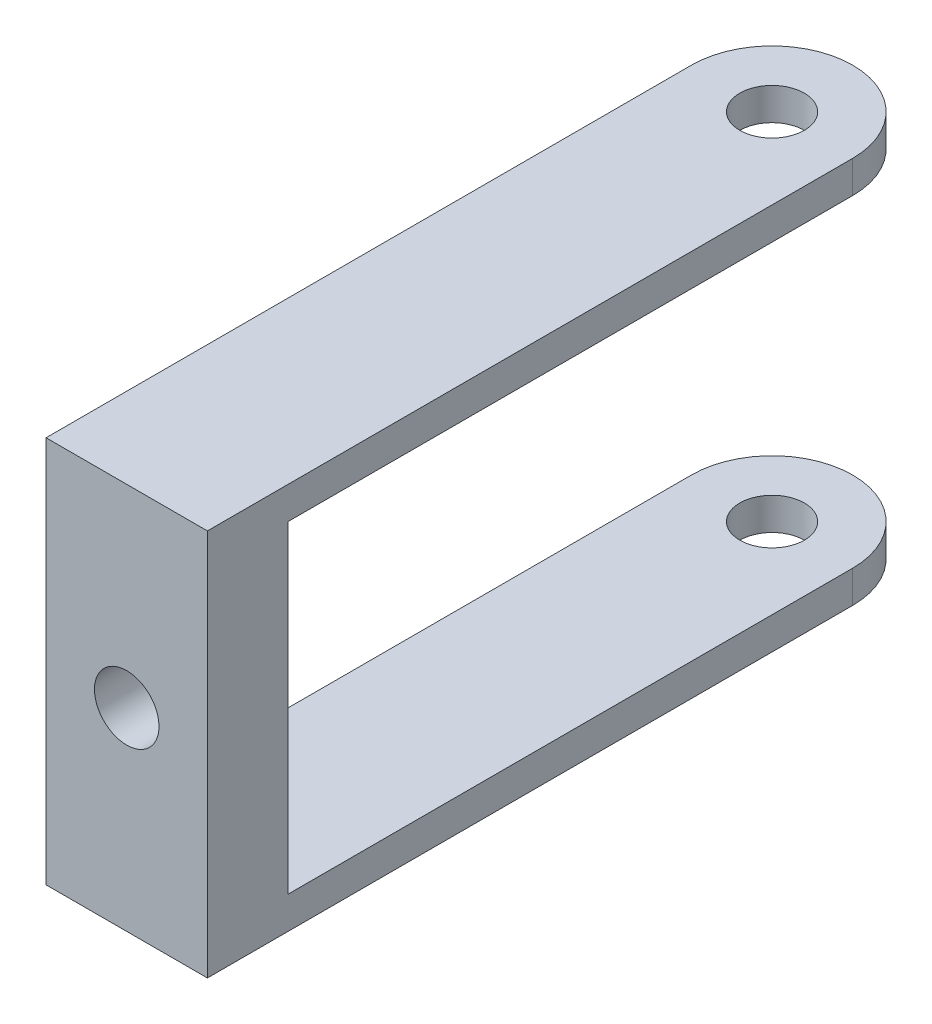
SolidWorks part; units mm, degrees
ref_plane "Front Plane" through (0, 0, 0) normal (0, 0, 1) x (1, 0, 0)
ref_plane "Top Plane" through (0, 0, 0) normal (0, 1, 0) x (1, 0, 0)
ref_plane "Right Plane" through (0, 0, 0) normal (1, 0, 0) x (0, 0, -1)
other "Configuration Table"
sketch "Sketch1" plane through (0, 0, 0) normal (0, 1, 0) x (1, 0, 0)
  line L0 (-5, 0) -> (-5, -40)
  line L1 (0, -3.85) -> (0, 3.85) construction
  line L2 (5, 0) -> (5, -40)
  line L3 (-5, -40) -> (5, -40)
  arc A0 (5, 0) -> (-5, 0) centre (0, 0) ccw
  dimension "D1" = 10
  dimension "D2" = 40
extrude "Boss-Extrude1" add sketch "Sketch1" along normal blind 24
sketch "Sketch2" plane through (0, 24, 0) normal (0, 1, 0) x (1, 0, 0)
  circle A0 centre (0, 0) radius 2
  dimension "D1" = 4
extrude "Cut-Extrude1" cut sketch "Sketch2" against normal through all both and the other way through all
sketch "Sketch3" plane through (5, 0, 0) normal (1, 0, 0) x (0, 0, -1)
  line L0 (-35, 22) -> (5, 22)
  line L1 (5, 0) -> (5, 24) construction
  line L2 (5, 22) -> (5, 2)
  line L3 (5, 2) -> (-35, 2)
  line L4 (-35, 2) -> (-35, 22)
  line L5 (-40, 24) -> (0, 24) construction
  line L6 (-40, 0) -> (0, 0) construction
  line L7 (-40, 24) -> (-40, 0) construction
  dimension "D1" = 2
  dimension "D2" = 2
  dimension "D3" = 5
extrude "Cut-Extrude2" cut sketch "Sketch3" against normal through all
sketch "Sketch4" plane through (0, 0, 35) normal (0, 0, -1) x (-1, 0, 0)
  line L0 (0, 24) -> (0, 0) construction
  line L1 (5, 24) -> (-5, 24) construction
  circle A0 centre (0, 12) radius 2
  dimension "D1" = 4
extrude "Cut-Extrude3" cut sketch "Sketch4" against normal through all
